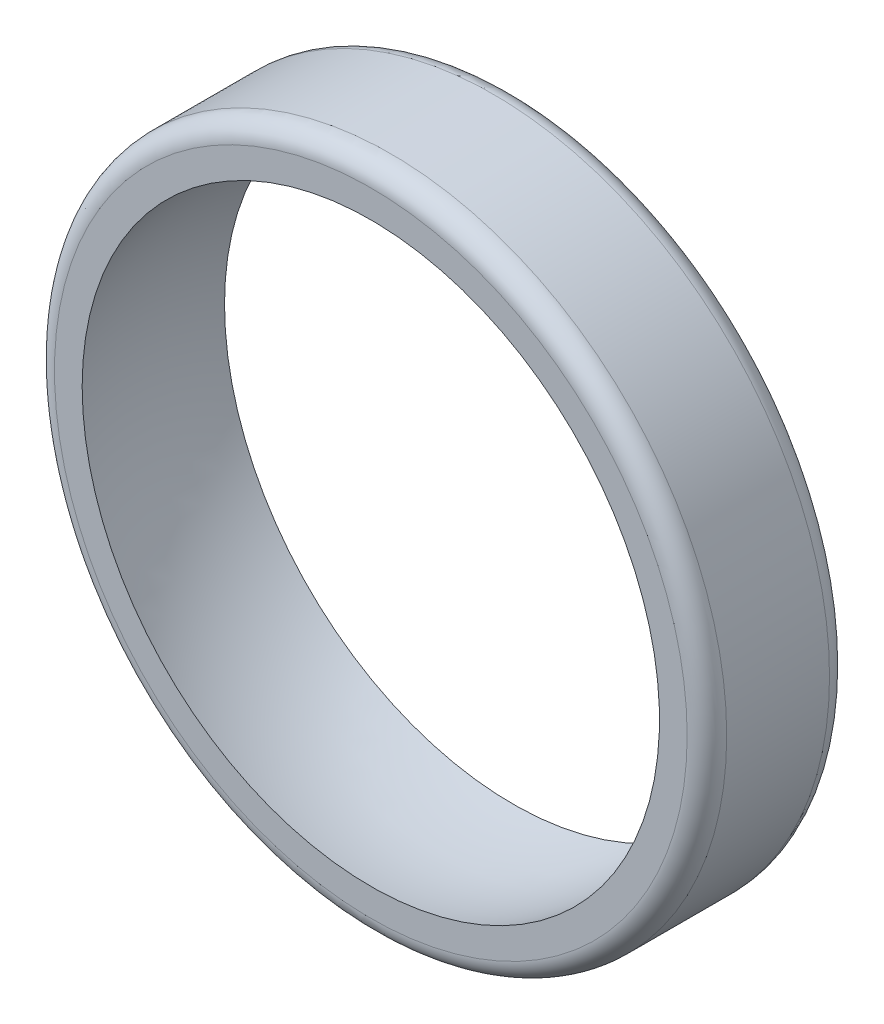
SolidWorks part; units mm, degrees
ref_plane "Front Plane" through (0, 0, 0) normal (0, 0, 1) x (1, 0, 0)
ref_plane "Top Plane" through (0, 0, 0) normal (0, 1, 0) x (1, 0, 0)
ref_plane "Right Plane" through (0, 0, 0) normal (1, 0, 0) x (0, 0, -1)
sketch "Sketch1" plane through (0, 0, 0) normal (0, 0, 1) x (1, 0, 0)
  circle A0 centre (0, 0) radius 42.5
  circle A1 centre (0, 0) radius 36.5
  dimension "D1" = 85
  dimension "D2" = 73
extrude "Boss-Extrude1" add sketch "Sketch1" along normal mid plane 18
sketch "Sketch2" plane through (0, 0, 0) normal (0, 1, 0) x (1, 0, 0)
  line L0 (42.5, 9) -> (36.5, 9) construction
  line L1 (42.5, 9) -> (-42.5, 9) construction
  line L2 (36.5, 9) -> (-36.5, 9) construction
  line L3 (36.5, 9) -> (36.5, -9)
  line L4 (-42.5, -9) -> (42.5, -9) construction
  line L5 (-36.5, -9) -> (36.5, -9) construction
  line L6 (36.5, -9) -> (42.5, -9) construction
  line L7 (0, 0) -> (0, -14.5289) construction
  line L8 (0, -9.9) -> (0, 9.9) construction
  arc A0 (36.5, 9) -> (36.5, -9) centre (-7.5908, 0) cw
  dimension "D1" = 45
revolve "Cut-Revolve1" cut sketch "Sketch2" angle 360 about L7
fillet "Fillet1" radius 2.5 2 edges at (42.5, 0, 9) (42.5, 0, -9)
